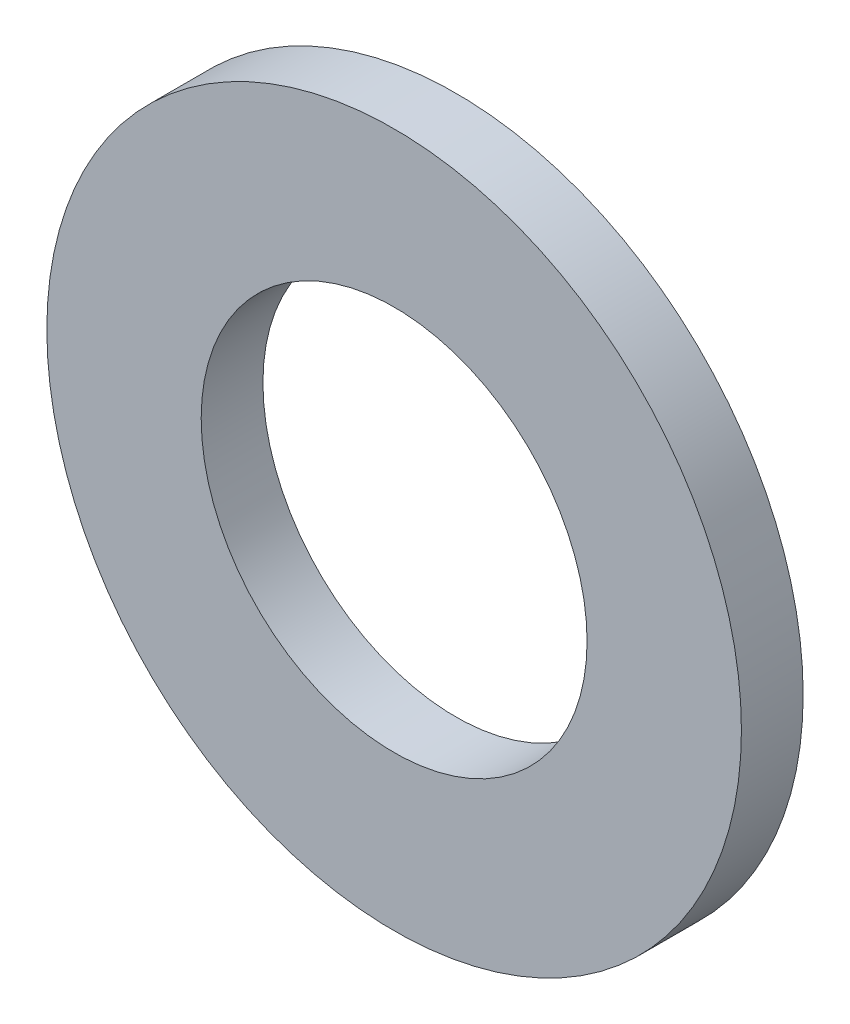
from build123d import *

# Parameters (mm, degrees)
SKETCH1_R           = 45
SKETCH1_R_2         = 25
BOSS_EXTRUDE1_DEPTH = 8
SKETCH2_R           = 42
SKETCH2_R_2         = 25
BOSS_EXTRUDE2_DEPTH = 3
SKETCH3_R           = 2.5
CUT_EXTRUDE1_DEPTH  = 6
CHAMFER1_SIZE       = 1
SKETCH4_R           = 42
SKETCH4_R_2         = 55
CUT_EXTRUDE2_DEPTH  = 3


with BuildPart() as part:
    # Sketch1 → Boss-Extrude1 (new body)
    with BuildSketch(Plane.XY):
        Circle(SKETCH1_R)
        Circle(SKETCH1_R_2, mode=Mode.SUBTRACT)
    extrude(amount=BOSS_EXTRUDE1_DEPTH)

    # Sketch2 → Boss-Extrude2 (add)
    with BuildSketch(Plane.XY.offset(8)):
        Circle(SKETCH2_R)
        Circle(SKETCH2_R_2, mode=Mode.SUBTRACT)
    extrude(amount=BOSS_EXTRUDE2_DEPTH)

    # Sketch3 → Cut-Extrude1 (cut)
    with BuildSketch(Plane(origin=(0, 0, 0), x_dir=(-1, 0, 0), z_dir=(0, 0, -1))):
        with Locations((0, 37)):
            Circle(SKETCH3_R)
        with Locations((32.04293994, 18.5)):
            Circle(SKETCH3_R)
        with Locations((32.04293994, -18.5)):
            Circle(SKETCH3_R)
        with Locations((0, -37)):
            Circle(SKETCH3_R)
        with Locations((-32.04293994, -18.5)):
            Circle(SKETCH3_R)
        with Locations((-32.04293994, 18.5)):
            Circle(SKETCH3_R)
    extrude(amount=-CUT_EXTRUDE1_DEPTH, mode=Mode.SUBTRACT)

    # Chamfer1
    chamfer1_edges = [part.edges().sort_by_distance(p)[0] for p in [
        (-42, 0, 11),
        (-25, 0, 11),
    ]]
    chamfer(chamfer1_edges, length=CHAMFER1_SIZE)

    # Sketch4 → Cut-Extrude2 (cut)
    with BuildSketch(Plane(origin=(248.99389391, -65.332745645, 8), x_dir=(0.8404902422792763, -0.5418266813597531, 0), z_dir=(0, 0, -1))):
        with Locations((-244.675962976, 80)):
            Circle(SKETCH4_R)
        with Locations((-244.675962976, -130)):
            Circle(SKETCH4_R_2)
    extrude(amount=-CUT_EXTRUDE2_DEPTH, mode=Mode.SUBTRACT)


solid = part.part
